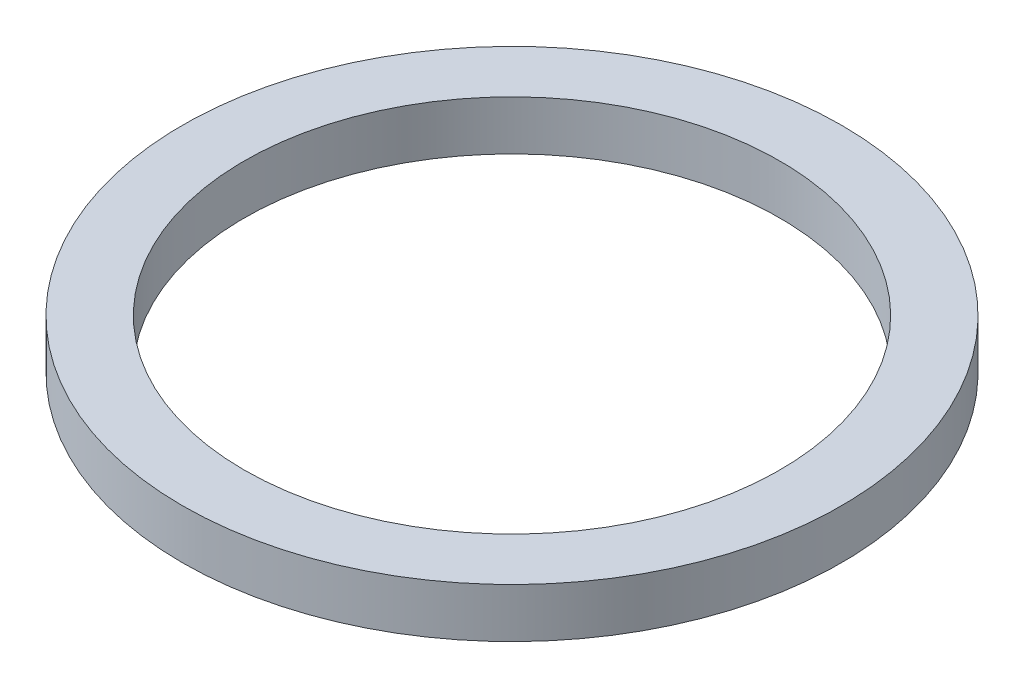
SolidWorks part; units mm, degrees
ref_plane "Front Plane" through (0, 0, 0) normal (0, 0, 1) x (1, 0, 0)
ref_plane "Top Plane" through (0, 0, 0) normal (0, 1, 0) x (1, 0, 0)
ref_plane "Right Plane" through (0, 0, 0) normal (1, 0, 0) x (0, 0, -1)
sketch "Sketch1" plane through (0, 0, 0) normal (0, 1, 0) x (1, 0, 0)
  circle A0 centre (0, 0) radius 32.5
  circle A1 centre (0, 0) radius 40
  dimension "D1" = 65
  dimension "D2" = 7.5
extrude "Boss-Extrude1" add sketch "Sketch1" along normal blind 6
